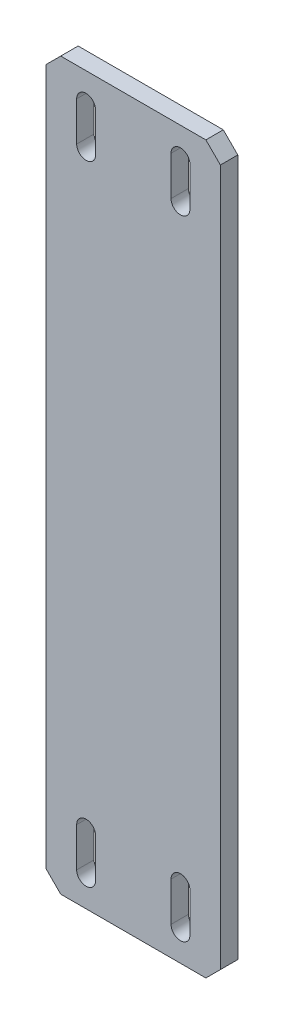
SolidWorks part; units mm, degrees
material "1023 碳钢板 (SS)"
ref_plane "Front Plane" through (0, 0, 0) normal (0, 0, 1) x (1, 0, 0)
ref_plane "Top Plane" through (0, 0, 0) normal (0, 1, 0) x (1, 0, 0)
ref_plane "Right Plane" through (0, 0, 0) normal (1, 0, 0) x (0, 0, -1)
sketch "Sketch1" plane through (0, 0, 0) normal (0, 0, 1) x (1, 0, 0)
  line L1 (-60, 250) -> (60, 250)
  line L2 (-60, 250) -> (-60, -250)
  line L3 (-60, -250) -> (60, -250)
  line L4 (60, 250) -> (60, -250)
  line L5 (-60, 250) -> (60, -250) construction
  line L6 (-60, -250) -> (60, 250) construction
  point P0 (0, 0)
  dimension "D1" = 120
  dimension "D2" = 500
extrude "Boss-Extrude1" add sketch "Sketch1" along normal blind 12
sketch "Sketch2" plane through (0, 0, 12) normal (0, 0, 1) x (1, 0, 0)
  line L0 (-32.5, 230) -> (-32.5, 203) construction
  line L1 (-26, 230) -> (-26, 203)
  line L2 (-39, 230) -> (-39, 203)
  line L3 (-60, 250) -> (-60, -250) construction
  line L4 (60, 250) -> (-60, 250) construction
  line L7 (32.5, 230) -> (32.5, 203) construction
  line L8 (26, 230) -> (26, 203)
  line L9 (39, 230) -> (39, 203)
  line L10 (32.5, -230) -> (32.5, -203) construction
  line L11 (26, -230) -> (26, -203)
  line L12 (39, -230) -> (39, -203)
  line L13 (-32.5, -230) -> (-32.5, -203) construction
  line L14 (-26, -230) -> (-26, -203)
  line L15 (-39, -230) -> (-39, -203)
  arc A0 (-26, 230) -> (-39, 230) centre (-32.5, 230) ccw
  arc A1 (-39, 203) -> (-26, 203) centre (-32.5, 203) ccw
  arc A2 (26, 230) -> (39, 230) centre (32.5, 230) cw
  arc A3 (39, 203) -> (26, 203) centre (32.5, 203) cw
  arc A4 (26, -230) -> (39, -230) centre (32.5, -230) ccw
  arc A5 (39, -203) -> (26, -203) centre (32.5, -203) ccw
  arc A6 (-26, -230) -> (-39, -230) centre (-32.5, -230) cw
  arc A7 (-39, -203) -> (-26, -203) centre (-32.5, -203) cw
  point P2 (-32.5, 216.5)
  point P18 (32.5, 216.5)
  point P25 (32.5, -216.5)
  point P32 (-32.5, -216.5)
  dimension "D1" = 27.5
  dimension "D2" = 6.5
  dimension "D3" = 20
  dimension "D4" = 27
  dimension "D5" = 27
  dimension "D6" = 27
  dimension "D7" = 27
  dimension "D8" = 406
extrude "Cut-Extrude1" cut sketch "Sketch2" against normal blind 12
chamfer "Chamfer1" distance 10 angle 45 4 edges at (60, -250, 6) (-60, -250, 6) (60, 250, 6) (-60, 250, 6)
